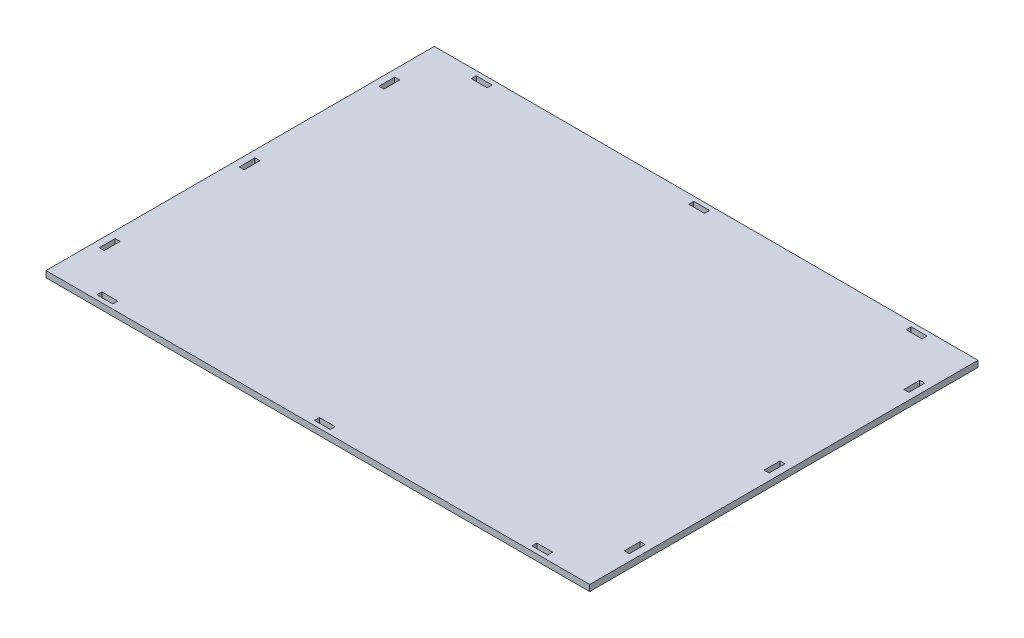
from build123d import *

# Parameters (mm, degrees)
SKETCH1_W           = 350
SKETCH1_H           = 250
BOSS_EXTRUDE1_DEPTH = 4
SKETCH2_W           = 3.2
SKETCH2_H           = 10.2
CUT_EXTRUDE1_DEPTH  = 216.095327704
SKETCH3_W           = 10.2
SKETCH3_H           = 3.2
CUT_EXTRUDE2_DEPTH  = 216.095327704


with BuildPart() as part:
    # Sketch1 → Boss-Extrude1 (new body)
    with BuildSketch(Plane(origin=(0, 0, 0), x_dir=(1, 0, 0), z_dir=(0, 1, 0))):
        Rectangle(SKETCH1_W, SKETCH1_H)
    extrude(amount=BOSS_EXTRUDE1_DEPTH)

    # Sketch2 → Cut-Extrude1 (cut, through all)
    with BuildSketch(Plane(origin=(0, 4, 0), x_dir=(1, 0, 0), z_dir=(0, 1, 0))):
        with Locations((-169, 90)):
            Rectangle(SKETCH2_W, SKETCH2_H)
        with Locations((-169, 0)):
            Rectangle(SKETCH2_W, SKETCH2_H)
        with Locations((-169, -90)):
            Rectangle(SKETCH2_W, SKETCH2_H)
        with Locations((169, -90)):
            Rectangle(SKETCH2_W, SKETCH2_H)
        with Locations((169, 0)):
            Rectangle(SKETCH2_W, SKETCH2_H)
        with Locations((169, 90)):
            Rectangle(SKETCH2_W, SKETCH2_H)
    extrude(amount=-CUT_EXTRUDE1_DEPTH, mode=Mode.SUBTRACT)

    # Sketch3 → Cut-Extrude2 (cut, through all)
    with BuildSketch(Plane(origin=(0, 4, 0), x_dir=(1, 0, 0), z_dir=(0, 1, 0))):
        with Locations((0, 120.5)):
            Rectangle(SKETCH3_W, SKETCH3_H)
        with Locations((140, 120.5)):
            Rectangle(SKETCH3_W, SKETCH3_H)
        with Locations((-140, 120.5)):
            Rectangle(SKETCH3_W, SKETCH3_H)
        with Locations((-140, -120.5)):
            Rectangle(SKETCH3_W, SKETCH3_H)
        with Locations((140, -120.5)):
            Rectangle(SKETCH3_W, SKETCH3_H)
        with Locations((0, -120.5)):
            Rectangle(SKETCH3_W, SKETCH3_H)
    extrude(amount=-CUT_EXTRUDE2_DEPTH, mode=Mode.SUBTRACT)


solid = part.part
